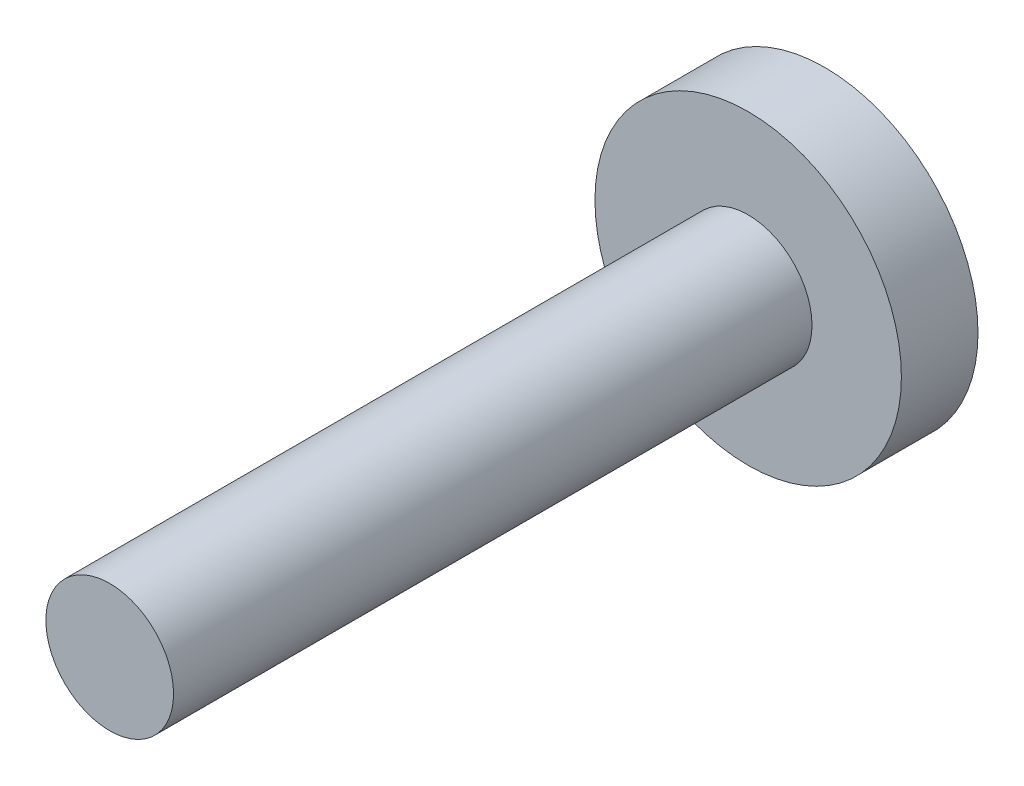
SolidWorks part; units mm, degrees
ref_plane "前视基准面" through (0, 0, 0) normal (0, 0, 1) x (1, 0, 0)
ref_plane "上视基准面" through (0, 0, 0) normal (0, 1, 0) x (1, 0, 0)
ref_plane "右视基准面" through (0, 0, 0) normal (1, 0, 0) x (0, 0, -1)
other "Configuration Table"
sketch "草图1" plane through (0, 0, 0) normal (0, 0, 1) x (1, 0, 0)
  circle A0 centre (0, 0) radius 5
  point P0 (0, 0)
  dimension "D1" = 10
extrude "凸台-拉伸1" add sketch "草图1" along normal blind 50
sketch "草图2" plane through (0, 0, 0) normal (0, 0, 1) x (1, 0, 0)
  circle A0 centre (0, 0) radius 12
  point P0 (0, 0)
  dimension "D1" = 24
extrude "凸台-拉伸2" add sketch "草图2" against normal blind 6
